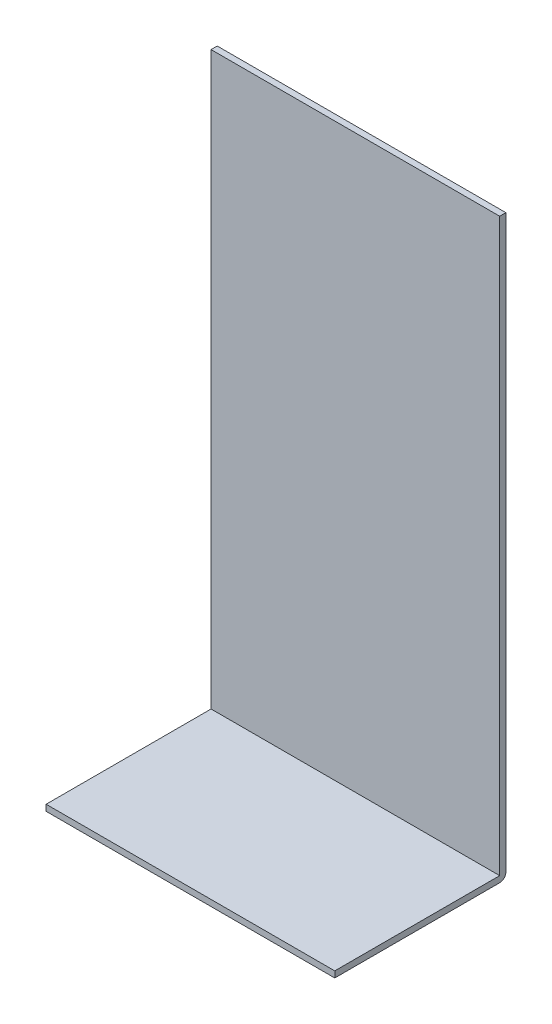
from build123d import *

# Parameters (mm, degrees)
SKETCH_1_W      = 140
SKETCH_1_H      = 280
EXTRUDE_1_DEPTH = 3
SKETCH_2_W      = 140
SKETCH_2_H      = 3
EXTRUDE_2_DEPTH = 80
FILLET_1_R      = 3


with BuildPart() as part:
    # 草图1 → 凸台-拉伸1 (new body)
    with BuildSketch(Plane.XY):
        with Locations((70, -140)):
            Rectangle(SKETCH_1_W, SKETCH_1_H)
    extrude(amount=EXTRUDE_1_DEPTH)

    # 草图2 → 凸台-拉伸2 (add)
    with BuildSketch(Plane.XY.offset(3)):
        with Locations((70, -278.5)):
            Rectangle(SKETCH_2_W, SKETCH_2_H)
    extrude(amount=EXTRUDE_2_DEPTH)

    # 圆角1
    fillet_1_edges = [part.edges().sort_by_distance(p)[0] for p in [
        (70, -280, 0),
    ]]
    fillet(fillet_1_edges, radius=FILLET_1_R)


solid = part.part
